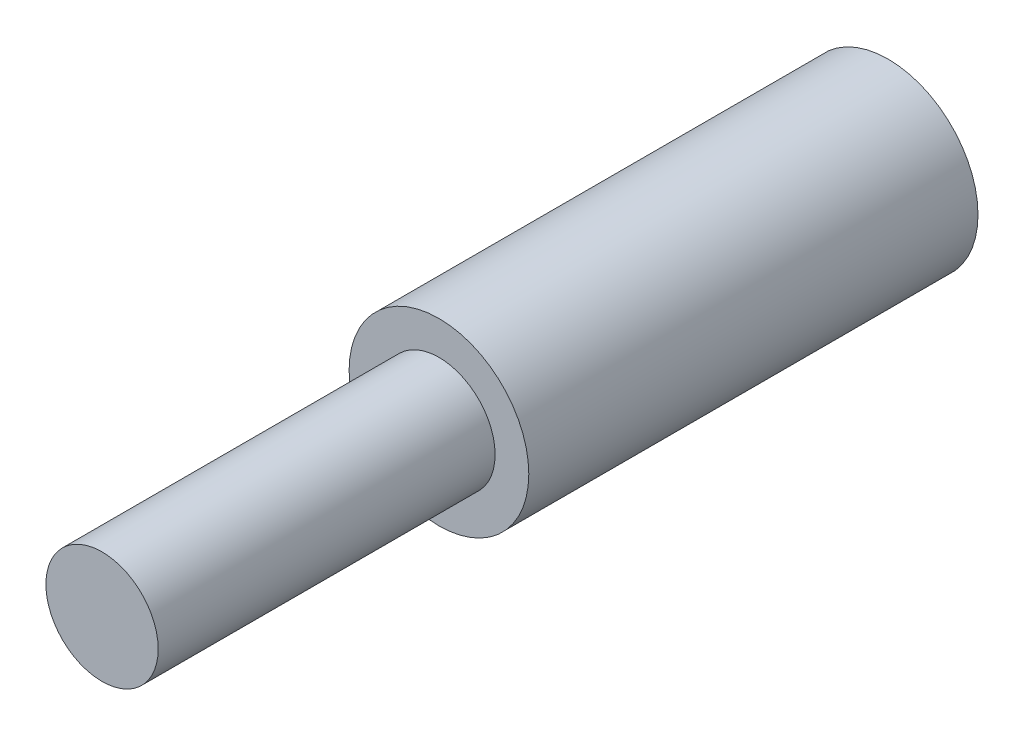
SolidWorks part; units mm, degrees
ref_plane "Front Plane" through (0, 0, 0) normal (0, 0, 1) x (1, 0, 0)
ref_plane "Top Plane" through (0, 0, 0) normal (0, 1, 0) x (1, 0, 0)
ref_plane "Right Plane" through (0, 0, 0) normal (1, 0, 0) x (0, 0, -1)
sketch "Sketch1" plane through (0, 0, 0) normal (0, 0, 1) x (1, 0, 0)
  circle A0 centre (0, 0) radius 8
extrude "Boss-Extrude1" add sketch "Sketch1" along normal blind 40
sketch "Sketch2" plane through (0, 0, 40) normal (0, 0, 1) x (1, 0, 0)
  circle A0 centre (0, 0) radius 5
extrude "Boss-Extrude2" add sketch "Sketch2" along normal blind 30
